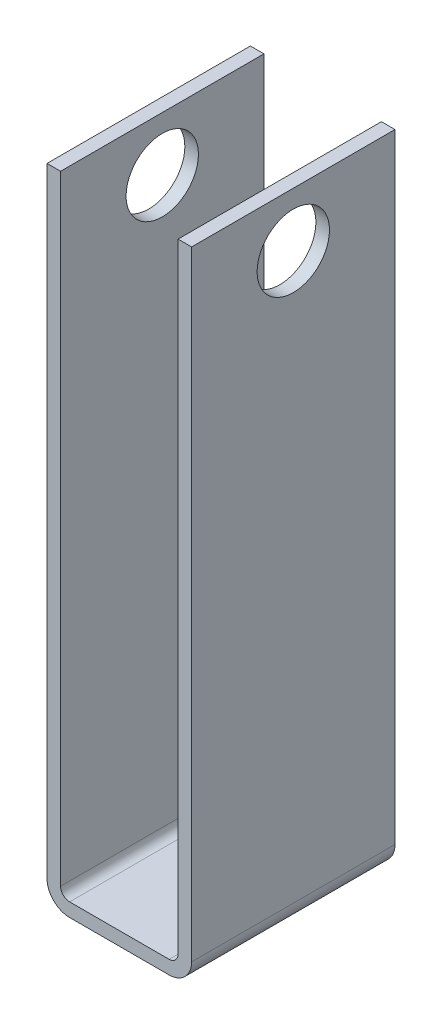
SolidWorks part; units mm, degrees
ref_plane "Front Plane" through (0, 0, 0) normal (0, 0, 1) x (1, 0, 0)
ref_plane "Top Plane" through (0, 0, 0) normal (0, 1, 0) x (1, 0, 0)
ref_plane "Right Plane" through (0, 0, 0) normal (1, 0, 0) x (0, 0, -1)
sketch "Sketch1" plane through (0, 0, 0) normal (0, 0, 1) x (1, 0, 0)
  line L0 (0, 0) -> (0, -137)
  line L1 (5, -142) -> (27, -142)
  line L2 (32, -137) -> (32, 0)
  line L3 (3, 0) -> (3, -137)
  line L4 (5, -139) -> (27, -139)
  line L5 (29, -137) -> (29, 0)
  line L6 (3, 0) -> (0, 0)
  line L7 (29, 0) -> (32, 0)
  arc A0 (27, -142) -> (32, -137) centre (27, -137) ccw
  arc A1 (0, -137) -> (5, -142) centre (5, -137) ccw
  arc A2 (3, -137) -> (5, -139) centre (5, -137) ccw
  arc A3 (27, -139) -> (29, -137) centre (27, -137) ccw
  point P8 (32, -142)
  point P11 (0, -142)
  dimension "D3" = 5
  dimension "D1" = 32
  dimension "D2" = 142
  dimension "D4" = 3
extrude "Boss-Extrude1" add sketch "Sketch1" along normal blind 45
sketch "Sketch2" plane through (32, 0, 0) normal (1, 0, 0) x (0, 0, -1)
  line L0 (0, -137) -> (0, 0) construction
  line L1 (-45, 0) -> (0, 0) construction
  circle A0 centre (-22.5, -12) radius 8
  dimension "D1" = 16
  dimension "D2" = 22.5
  dimension "D3" = 12
extrude "Cut-Extrude1" cut sketch "Sketch2" against normal through all
